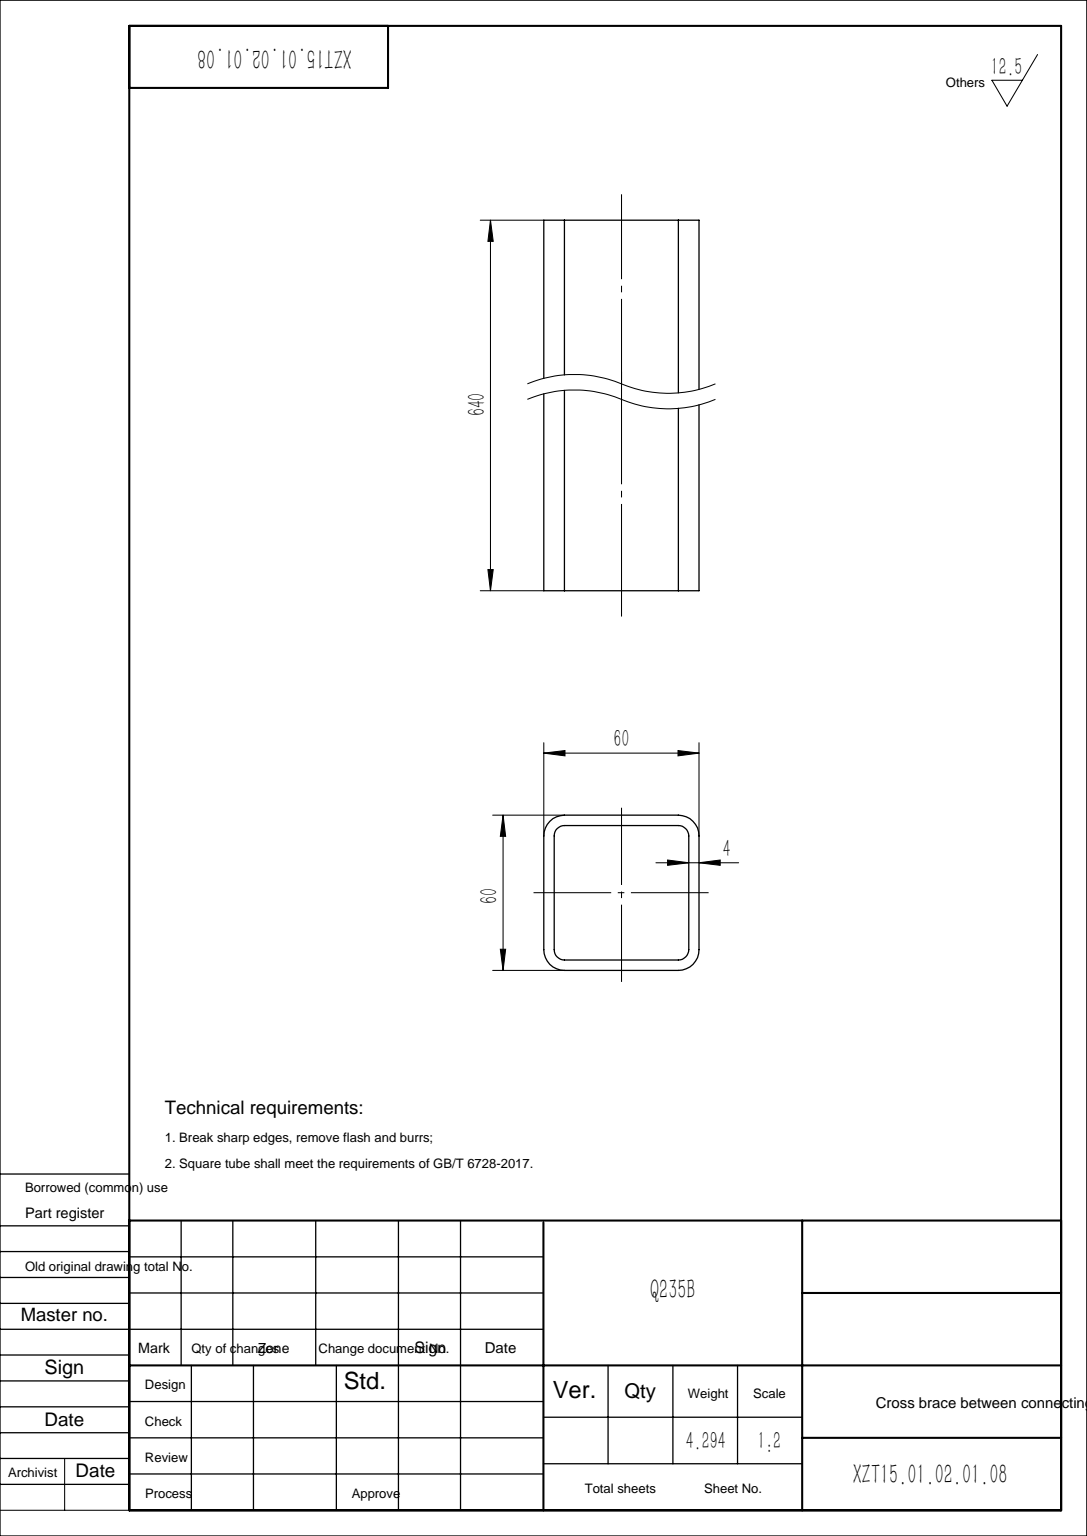
from build123d import *

# Parameters (mm, degrees)
GB_T_6728_2002_SQUARE_HOLLOW_SECTION_60_DEPTH = 640


with BuildPart() as part:
    # Sketch1 → GB/T 6728-2002 square hollow section 60×60×4(1) (new body)
    with BuildSketch(Plane(origin=(0, 0, 0), x_dir=(-1, 0, 0), z_dir=(0, 1, 0))):
        with BuildLine():
            Line((-22, -30), (22, -30))
            ThreePointArc((22, -30), (27.656854249, -27.656854249), (30, -22))
            Line((30, -22), (30, 22))
            ThreePointArc((30, 22), (27.656854249, 27.656854249), (22, 30))
            Line((22, 30), (-22, 30))
            ThreePointArc((-22, 30), (-27.656854249, 27.656854249), (-30, 22))
            Line((-30, 22), (-30, -22))
            ThreePointArc((-30, -22), (-27.656854249, -27.656854249), (-22, -30))
        make_face()
        with BuildLine():
            Line((-22, -26), (22, -26))
            ThreePointArc((22, -26), (24.828427125, -24.828427125), (26, -22))
            Line((26, -22), (26, 22))
            ThreePointArc((26, 22), (24.828427125, 24.828427125), (22, 26))
            Line((22, 26), (-22, 26))
            ThreePointArc((-22, 26), (-24.828427125, 24.828427125), (-26, 22))
            Line((-26, 22), (-26, -22))
            ThreePointArc((-26, -22), (-24.828427125, -24.828427125), (-22, -26))
        make_face(mode=Mode.SUBTRACT)
    extrude(amount=GB_T_6728_2002_SQUARE_HOLLOW_SECTION_60_DEPTH)


solid = part.part
